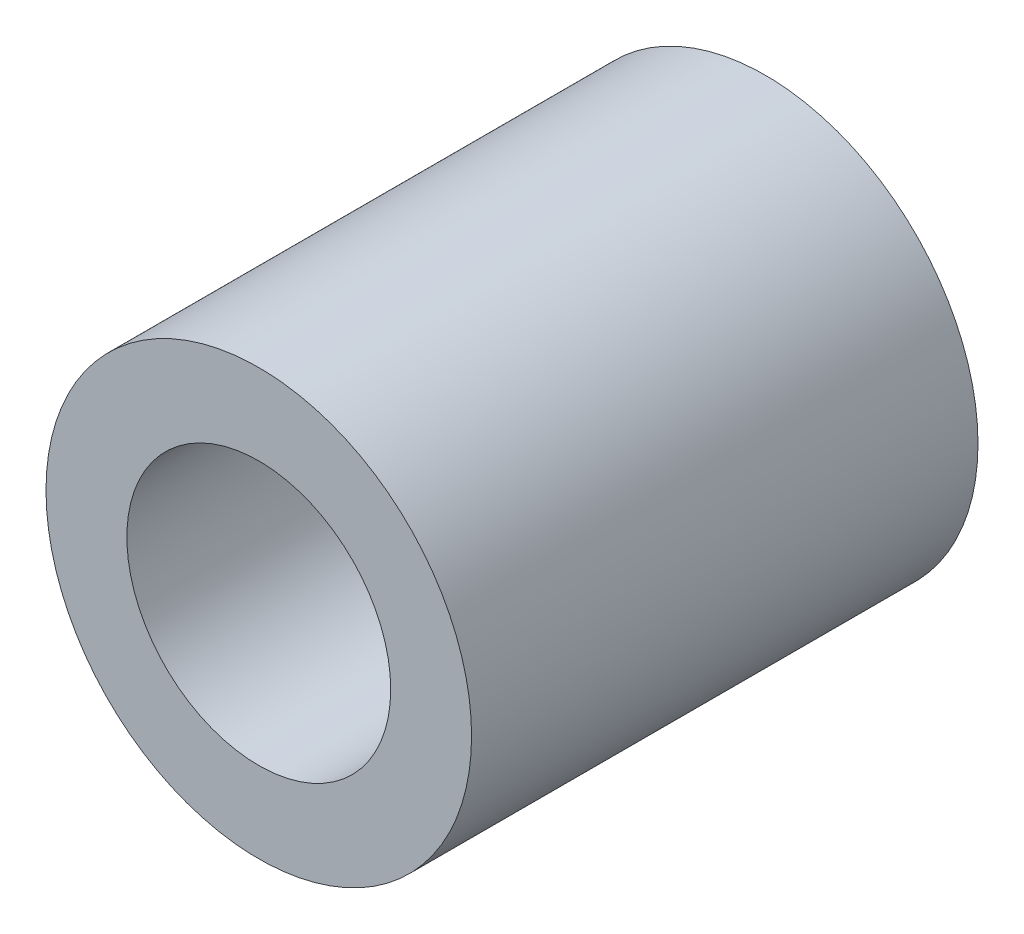
from build123d import *

# Parameters (mm, degrees)
SKETCH_1_R      = 2.5
SKETCH_1_R_2    = 1.55
EXTRUDE_1_DEPTH = 5.95


with BuildPart() as part:
    # 草图1 → 凸台-拉伸1 (new body)
    with BuildSketch(Plane.XY):
        Circle(SKETCH_1_R)
        Circle(SKETCH_1_R_2, mode=Mode.SUBTRACT)
    extrude(amount=EXTRUDE_1_DEPTH)


solid = part.part
